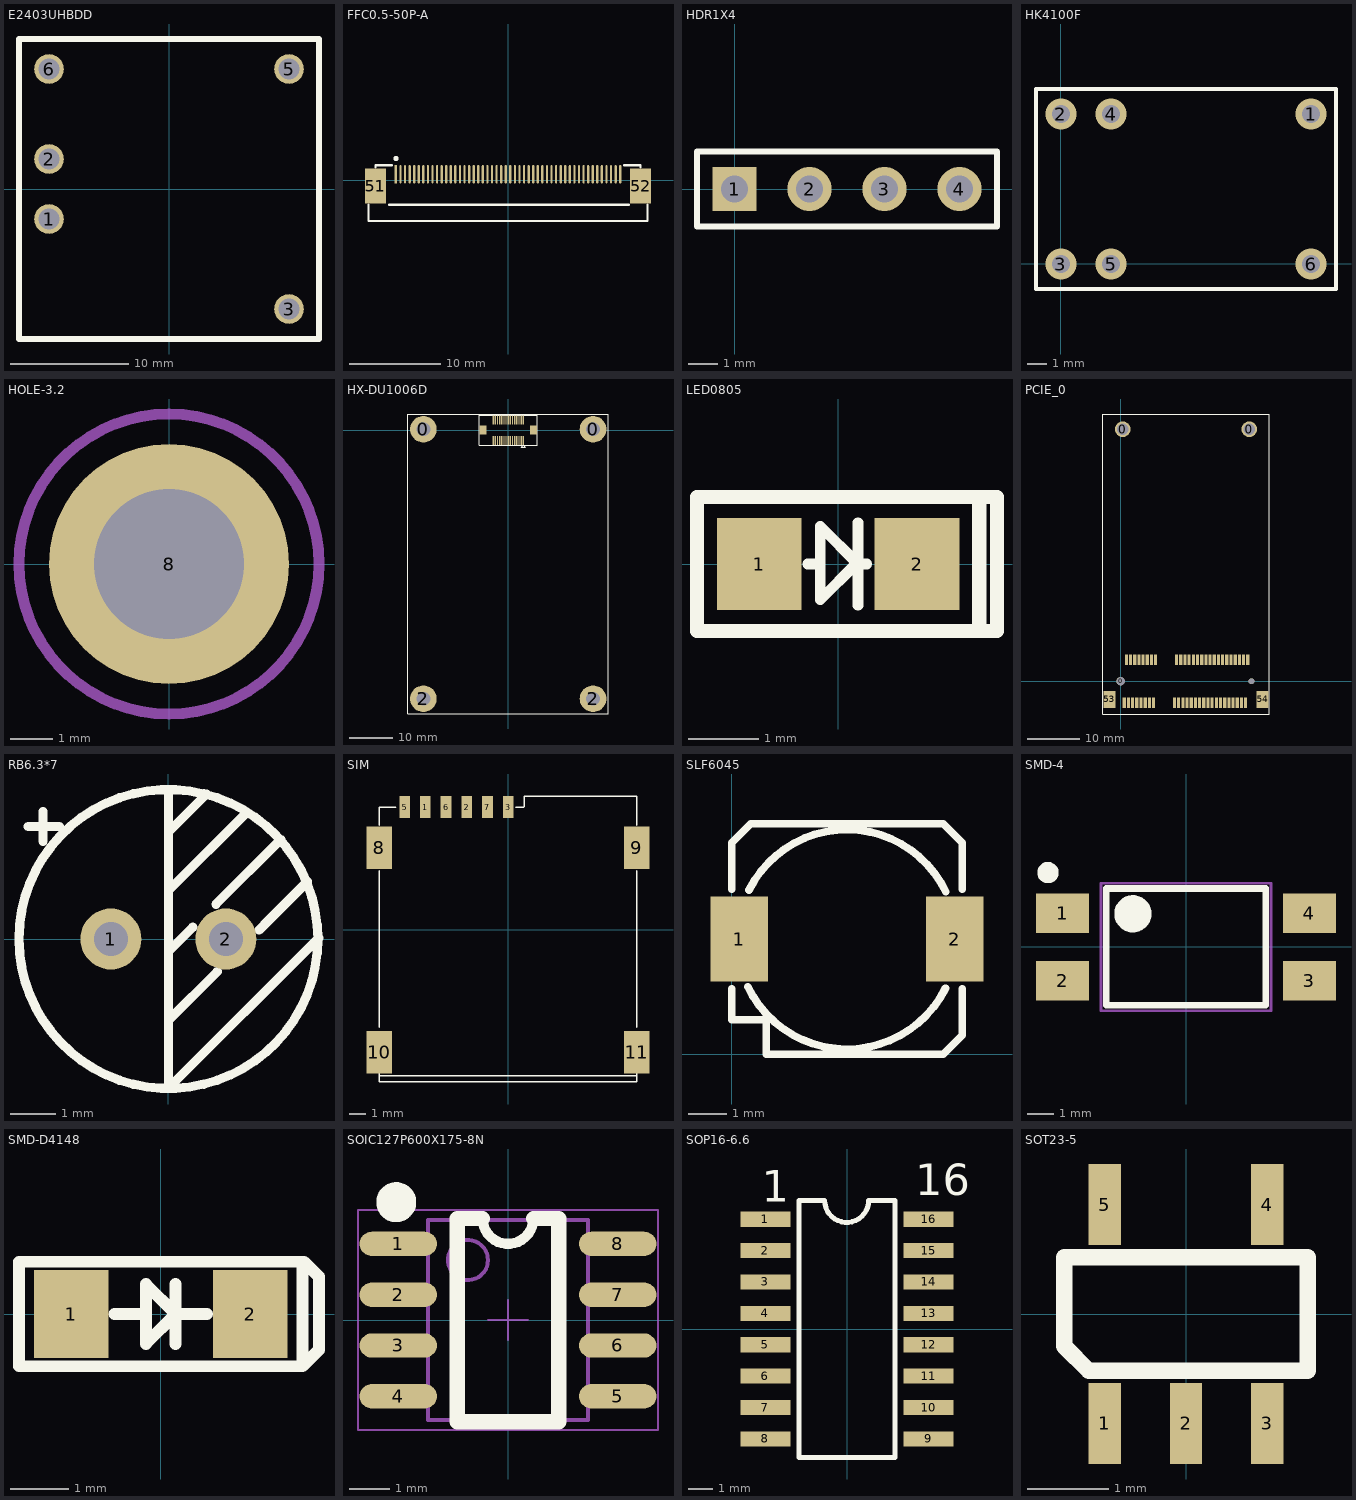
[diagram p0: the footprints below, top view; thin cyan lines are the x and y axes]
# Altium footprint library MISC82794-2.PcbLib: 41 footprints (part 2 of 3)
Each footprint in its own frame and in the unit in brackets; x right, y up, seen from the top. Pads: shape width x height; smd on the part's side, far side on the other; paste and mask are expansions set on the pad; w line width, h text height; cw(c..) or ccw(c..) is an arc to the next point about the centre after c.

## E2403UHBDD [mm]
height 9.5
pads (5):
  round 2.5 hole 1.8: 1(-10.16,-2.54) 2(-10.16,2.54) 3(10.16,-10.16) 5(10.16,10.16) 6(-10.16,10.16)
Top Overlay:
  lines w0.5: -12.7,-12.7 -12.7,12.7 12.7,12.7 12.7,-12.7 -12.7,-12.7

## FFC0.5-50P-A [mm]
height 9.5
pads (52):
  rect 0.25x2 smd: 1(-12.246,0.645)
  oval 0.25x2 smd: 2(-11.746,0.645) 3(-11.246,0.645) 4(-10.746,0.645) 5(-10.246,0.645) 6(-9.746,0.645) 7(-9.246,0.645) 8(-8.746,0.645) 9(-8.246,0.645) 10(-7.746,0.645) 11(-7.246,0.645) 12(-6.746,0.645) 13(-6.246,0.645) 14(-5.746,0.645) 15(-5.246,0.645) 16(-4.746,0.645) 17(-4.246,0.645) 18(-3.746,0.645) 19(-3.246,0.645) 20(-2.746,0.645) 21(-2.246,0.645) 22(-1.746,0.645) 23(-1.246,0.645) 24(-0.746,0.645) 25(-0.246,0.645) 26(0.254,0.645) 27(0.754,0.645) 28(1.254,0.645) 29(1.754,0.645) 30(2.254,0.645) 31(2.754,0.645) 32(3.254,0.645) 33(3.754,0.645) 34(4.254,0.645) 35(4.754,0.645) 36(5.254,0.645) 37(5.754,0.645) 38(6.254,0.645) 39(6.754,0.645) 40(7.254,0.645) 41(7.754,0.645) 42(8.254,0.645) 43(8.754,0.645) 44(9.254,0.645) 45(9.754,0.645) 46(10.254,0.645) 47(10.754,0.645) 48(11.254,0.645) 49(11.754,0.645) 50(12.254,0.645)
  rect 2.286x3.81 smd: 51(-14.478,-0.645) 52(14.478,-0.645)
Top Overlay:
  circle w0.254: c-12.228,2.362 r0.163
  lines w0.254: -15.24,-2.677 -15.24,-4.455 15.24,-4.455 15.24,-2.677 ; -14.478,1.387 -14.478,1.641 -12.7,1.641 ; -12.954,-2.677 13.208,-2.677 ; 12.7,1.641 14.478,1.641 14.478,1.387

## HDR1X4 [mm] "Connector; Header; 4 Position"
pads (4):
  rect 1.5x1.5 hole 0.9: 1(0,0)
  round 1.5 hole 0.9: 2(2.54,0) 3(5.08,0) 4(7.62,0)
Top Overlay:
  lines w0.2: -1.27,-1.27 -1.27,1.27 8.89,1.27 8.89,-1.27 -1.27,-1.27

## HK4100F [mm] "11.8mm"
height 9.5
pads (6):
  round 1.6 hole 0.9: 1(12.7,7.62) 2(0,7.62) 3(0,0) 4(2.54,7.62) 5(2.54,0) 6(12.7,0)
Top Overlay:
  lines w0.2: -1.27,-1.27 13.97,-1.27 13.97,8.89 -1.27,8.89 -1.27,-1.27

## HOLE-3.2 [mm]
height 9.5
pads (1):
  round 5.6 hole 3.5: 8(0,0)
Mechanical 15:
  circle w0.254: c0,0 r3.5

## HX-DU1006D [mm]
pads (36):
  round 6.2 hole 3.2: 0(-19.75,0.23) 0(19.75,0.23) 2(-19.75,-62.51) 2(19.75,-62.51)
  rect 0.3x2.1 smd: 1(3.5,-2.35) 2(3.5,2.35) 3(3,-2.35) 4(3,2.35) 5(2.5,-2.35) 6(2.5,2.35) 7(2,-2.35) 8(2,2.35) 9(1.5,-2.35) 10(1.5,2.35) 11(1,-2.35) 12(1,2.35) 13(0.5,-2.35) 14(0.5,2.35) 15(0,-2.35) 16(0,2.35) 17(-0.5,-2.35) 18(-0.5,2.35) 19(-1,-2.35) 20(-1,2.35) 21(-1.5,-2.35) 22(-1.5,2.35) 23(-2,-2.35) 24(-2,2.35) 25(-2.5,-2.35) 26(-2.5,2.35) 27(-3,-2.35) 28(-3,2.35) 29(-3.5,-2.35) 30(-3.5,2.35)
  rect 1.6x2.1 smd: 31(-5.9,0) 31(5.9,0)
Top Overlay:
  lines w0.1: 3.476,-3.491 3.039,-3.928 3.928,-3.928 3.491,-3.491 ; -23.36,-66.07 -23.36,3.78 23.25,3.78 23.25,-66.07 -23.36,-66.07 ; -6.8,-3.5 6.8,-3.5 6.8,3.5 -6.8,3.5 -6.8,-3.5

## LED0805 [mm]
pads (2):
  rect 1.2x1.3 smd: 1(-1.118,0) 2(1.118,0)
Top Overlay:
  lines w0.152: -0.432,0 -0.254,0 ; 0.279,-0.584 0.279,0.584 ; 0.406,0 0.254,0 ; 0.254,0 -0.254,-0.508 -0.254,0.533 0.279,0 0.254,0
  lines w0.203: 1.93,-0.95 2.25,-0.95 2.25,0.95 2,0.95 ; 2,0.95 2,-0.95 -2,-0.95 -2,0.95 2,0.95

## PCIE_0 [mm]
height 3.98
pads (58):
  round 1.6 hole 1.6 unplated: 0(0,0)
  round 3 hole 2.2 unplated: 0(0.4,48.15) 0(24.6,48.15)
  round 1.1 hole 1.1 unplated: 0(25,0)
  rect 0.6x2 smd: 1(0.7,-4.1) 2(1.1,4.1) 3(1.5,-4.1) 4(1.9,4.1) 5(2.3,-4.1) 6(2.7,4.1) 7(3.1,-4.1) 8(3.5,4.1) 9(3.9,-4.1) 10(4.3,4.1) 11(4.7,-4.1) 12(5.1,4.1) 13(5.5,-4.1) 14(5.9,4.1) 15(6.3,-4.1) 16(6.7,4.1) 17(10.3,-4.1) 18(10.7,4.1) 19(11.1,-4.1) 20(11.5,4.1) 21(11.9,-4.1) 22(12.3,4.1) 23(12.7,-4.1) 24(13.1,4.1) 25(13.5,-4.1) 26(13.9,4.1) 27(14.3,-4.1) 28(14.7,4.1) 29(15.1,-4.1) 30(15.5,4.1) 31(15.9,-4.1) 32(16.3,4.1) 33(16.7,-4.1) 34(17.1,4.1) 35(17.5,-4.1) 36(17.9,4.1) 37(18.3,-4.1) 38(18.7,4.1) 39(19.1,-4.1) 40(19.5,4.1) 41(19.9,-4.1) 42(20.3,4.1) 43(20.7,-4.1) 44(21.1,4.1) 45(21.5,-4.1) 46(21.9,4.1) 47(22.3,-4.1) 48(22.7,4.1) 49(23.1,-4.1) 50(23.5,4.1) 51(23.9,-4.1) 52(24.3,4.1)
  rect 2.3x3.2 smd: 53(-2.15,-3.5) 54(27.15,-3.5)
Top Overlay:
  lines w0.1: -3.429,-6.275 -3.429,51.054 28.448,51.054 28.448,-6.275 -3.429,-6.275

## RB6.3*7 [mm]
pads (2):
  round 1.35 hole 0.75: 1(-1.27,0) 2(1.27,0)
Top Overlay:
  circle w0.203: c0,0 r3.302
  lines w0.203: -3.099,2.489 -2.413,2.489 ; -2.769,2.159 -2.769,2.819 ; 0,-1.8 1.079,-0.721 ; 0,-0.3 0,-0.28 0.539,0.259 ; 0,1.067 1.727,2.794 ; 0,2.362 0.838,3.2 ; 0,3.302 0,-3.302 3.327,0.025 ; 1.049,0.769 2.48,2.2 ; 2.003,0.2 3.073,1.27 2.134,0.33 2.13,0.33

## SIM [mm]
height 3.98
pads (10):
  rect 0.65x1.35 smd: 1(-5.07,7.512) 2(-2.53,7.512) 3(0.01,7.512) 5(-6.34,7.512) 6(-3.8,7.512) 7(-1.26,7.512)
  rect 1.55x2.6 smd: 8(-7.9,5.008) 9(7.9,5.008) 10(-7.9,-7.512) 11(7.9,-7.512)
Top Overlay:
  lines w0.1: -7.9,-8.962 7.9,-8.962 ; -7.9,-7.512 -7.9,-9.343 7.9,-9.343 7.9,-7.512 ; -7.9,-5.993 -7.9,3.611 ; -7.9,6.405 -7.9,7.512 -6.884,7.512 ; 0.482,7.512 0.955,7.512 0.99,7.548 0.99,8.183 7.9,8.183 7.9,6.405 ; 7.9,-5.993 7.9,3.611

## SLF6045 [mm]
height 3.98
pads (2):
  rect 1.5x2.2 smd: 1(0.2,3) 2(5.8,3)
Top Overlay:
  lines w0.2: 0,1.7 0,0.9 0.9,0.9 0.9,0 5.5,0 6,0.5 6,1.7 ; 0,4.3 0,5.5 0.5,6 5.5,6 6,5.5 6,4.3 ; 0.418,1.761 ccw(c3,3) 5.561,1.719 ; 0.454,4.273 cw(c3,3) 5.566,4.232

## SMD-4 [mm]
height 9.5
pads (4):
  rect 2x1.5 smd: 1(-4.65,1.27) 2(-4.65,-1.27) 3(4.65,-1.27) 4(4.65,1.27)
Top Overlay:
  circle w0.4: c-5.2,2.8 r0.2
  circle w0.7: c-2,1.25 r0.35
  lines w0.254: -3,-2.2 -3,2.2 3,2.2 3,-2.2 -3,-2.2
Mechanical 13:
  lines w0.1: -3.2,-2.4 3.2,-2.4 3.2,2.4 -3.2,2.4 -3.2,-2.4
3D body: height 3.9, standoff 0, extent -5.015,-2.416 5.015,2.416

## SMD-D4148 [mm]
pads (2):
  rect 1.27x1.5 smd: 1(-1.524,0) 2(1.524,0)
Top Overlay:
  lines w0.203: -0.787,0 -0.254,0 ; 0.254,-0.508 0.254,0.508 ; 0.787,0 0.254,0 ; 0.254,0 -0.254,-0.508 -0.254,0.508 0.254,0 ; 2.413,-0.889 2.692,-0.61 2.692,0.635 2.438,0.889 2.413,0.889 ; 2.413,-0.889 2.413,0.889 ; 2.413,-0.889 -2.413,-0.889 -2.413,0.889 2.413,0.889

## SOIC127P600X175-8N [mil]
height 374.02
pads (8):
  oval 76.06x24 smd: 1(-108.03,75) 2(-108.03,25) 3(-108.03,-25) 4(-108.03,-75) 5(108.03,-75) 6(108.03,-25) 7(108.03,25) 8(108.03,75)
Top Overlay:
  circle w23.62: c-110,116 r7.87
  lines w10: -25,100 ccw(c0,100) 25,100
  lines w15: -25,100 -50,100 -50,-100 50,-100 50,100 25,100
Mechanical 15:
  circle w3.94: c-39.37,59.06 r19.68
  lines w3.94: -78.74,-98.43 78.74,-98.43 78.74,98.43 -78.74,98.43 -78.74,-98.43
  text "1" at 17.71,-6.47 h50
Mechanical 16:
  lines w0.04: -78.74,-98.43 78.74,-98.43 78.74,98.43 -78.74,98.43 -78.74,-98.43
  lines w1.97: -19.68,0 19.68,0 ; 0,-19.68 0,19.68 ; -147.64,-108.27 147.64,-108.27 147.64,108.27 -147.64,108.27 -147.64,-108.27
3D body: height 61.02, standoff -1.97, extent -117.91,-96 117.91,96.91

## SOP16-6.6 [mil]
height 374.02
pads (16):
  rect 80x24 smd: 1(-130,175) 2(-130,125) 3(-130,75) 4(-130,25) 5(-130,-25) 6(-130,-75) 7(-130,-125) 8(-130,-175) 9(130,-175) 10(130,-125) 11(130,-75) 12(130,-25) 13(130,25) 14(130,75) 15(130,125) 16(130,175)
Top Overlay:
  lines w8: -76.5,-205 -76.5,205 -35.59,205 ccw(c-0.5,205) 34.59,205 76.5,205 76.5,-205 -76.5,-205
  text "1" at -136,203 h50
  text "16" at 109,213 h50

## SOT23-5 [mm]
height 9.5
pads (5):
  rect 0.4x1 smd: 1(-1,-1.35) 2(0,-1.35) 3(1,-1.35) 4(1,1.35) 5(-1,1.35)
Top Overlay:
  lines w0.203: -1.5,-0.4 -1.2,-0.7 1.5,-0.7 1.5,-0.6 1.5,0.7 0,0.7 -1.5,0.7 -1.5,-0.3 -1.5,-0.4